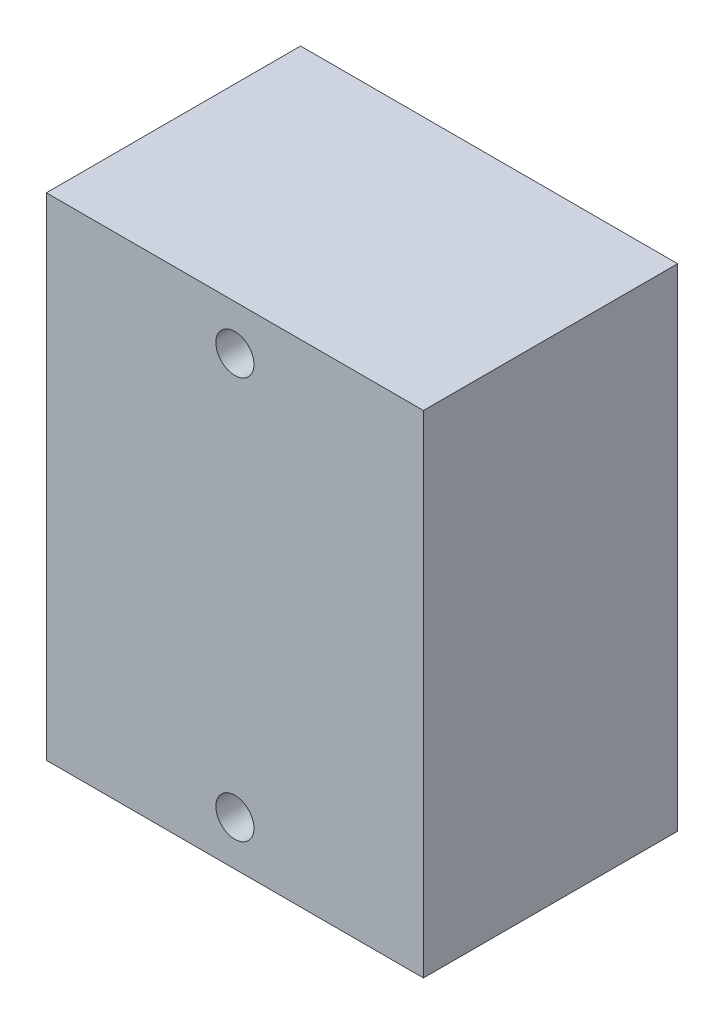
from build123d import *

# Parameters (mm, degrees)
SKETCH_1_W      = 44.5
SKETCH_1_H      = 58
SKETCH_1_R      = 2.25
EXTRUDE_1_DEPTH = 30


with BuildPart() as part:
    # 草图1 → 凸台-拉伸1 (new body)
    with BuildSketch(Plane.XY):
        Rectangle(SKETCH_1_W, SKETCH_1_H)
        with Locations((0, 23.7)):
            Circle(SKETCH_1_R, mode=Mode.SUBTRACT)
        with Locations((0, -23.7)):
            Circle(SKETCH_1_R, mode=Mode.SUBTRACT)
    extrude(amount=EXTRUDE_1_DEPTH)


solid = part.part
